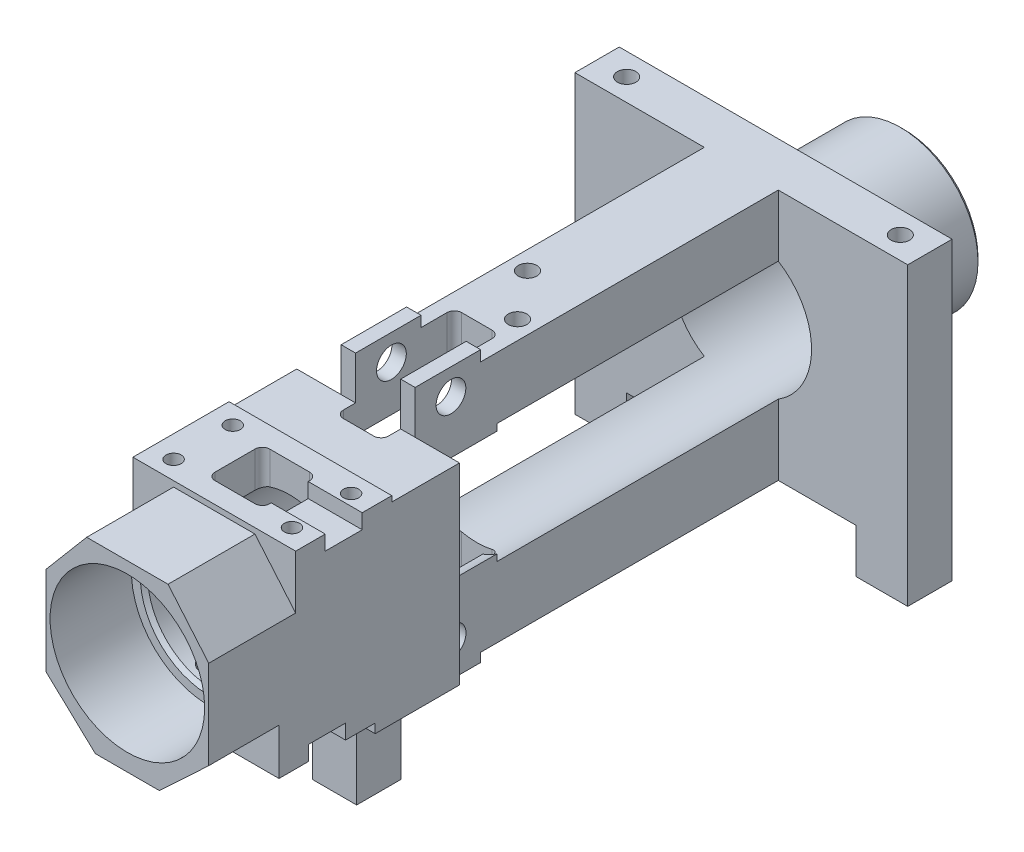
from build123d import *

# Parameters (mm, degrees)
SKETCH_1_R                   = 10.5
EXTRUDE_1_DEPTH              = 16
SKETCH_2_W                   = 45
SKETCH_2_H                   = 40
EXTRUDE_2_DEPTH              = 6
SKETCH_3_W                   = 10
SKETCH_3_H                   = 40
EXTRUDE_3_DEPTH              = 59
SKETCH_4_W                   = 22
SKETCH_4_H                   = 9.9
EXTRUDE_4_DEPTH              = 40
SKETCH_5_W                   = 8.85
SKETCH_5_H                   = 1.44
EXTRUDE_5_DEPTH              = 10
SKETCH_6_R                   = 8.75
CUT_EXTRUDE_1_DEPTH          = 88.316722339
SKETCH_7_W                   = 22
SKETCH_7_H                   = 4.4
SKETCH_7_H_2                 = 9.6
CUT_EXTRUDE_2_DEPTH          = 9.9
SKETCH_8_W                   = 6.1
SKETCH_8_H                   = 16
CUT_EXTRUDE_3_DEPTH          = 94.725789407
SKETCH_9_W                   = 10
SKETCH_9_H                   = 4.8
CUT_EXTRUDE_4_DEPTH          = 13.35
SKETCH_10_W                  = 31
SKETCH_10_H                  = 6
CUT_EXTRUDE_5_DEPTH          = 29.4
HOLE_WIZARD_M3_1_D           = 2.5
HOLE_WIZARD_M3_1_DEPTH       = 5
HOLE_WIZARD_M3_1_TIP         = 0.751075774
CUT_EXTRUDE_6_REACH          = 90.737
SKETCH_14_R                  = 2.01
SKETCH_14_R_2                = 2.03
HOLE_WIZARD_M3_2_D           = 2.5
HOLE_WIZARD_M3_2_DEPTH       = 5
HOLE_WIZARD_M3_2_TIP         = 0.751075774
SKETCH_18_R                  = 9.5
CUT_EXTRUDE_7_DEPTH          = 60
CHAMFER_1_SIZE               = 0.5
FILLET_1_R                   = 1
FILLET_2_R                   = 1
SKETCH_24_W                  = 10
SKETCH_24_H                  = 16.85
CUT_EXTRUDE_8_DEPTH          = 6
EXTRUDE_START                = 24
SKETCH_25_W                  = 22
SKETCH_25_H                  = 26
SKETCH_25_R                  = 8.75
EXTRUDE_8_DEPTH              = 24
SKETCH_26_R                  = 10.45
CUT_EXTRUDE_9_DEPTH          = 11
CHAMFER_5_SIZE               = 0.5
SKETCH_27_W                  = 6
SKETCH_27_H                  = 6
SKETCH_27_R                  = 1.2
EXTRUDE_9_DEPTH              = 9.6
HOLE_WIZARD_M3_5_D           = 2.5
HOLE_WIZARD_M3_5_DEPTH       = 9.6
HOLE_WIZARD_M3_5_TIP         = 0.751075774
SKETCH_41_W                  = 22
SKETCH_41_H                  = 13
SKETCH_41_R                  = 1
EXTRUDE_9959_DEPTH           = 0.75
CUT_EXTRUDE_START            = -12
CUT_EXTRUDE_10346_DEPTH      = 12
HOLE_WIZARD_10393_D          = 2.05
HOLE_WIZARD_10393_DEPTH      = 6.2
HOLE_WIZARD_10393_TIP        = 0.615882135
SKETCH_51_W                  = 7.3
SKETCH_51_H                  = 5
CUT_EXTRUDE_11630_DEPTH      = 2
SKETCH_47_R                  = 1
CUT_EXTRUDE_12263_DEPTH      = 1.25
CUT_EXTRUDE_12654_REACH      = 114.005
CUT_EXTRUDE_12654_END_RADIUS = 8.75
HOLE_WIZARD_12700_D          = 2.05
HOLE_WIZARD_12700_DEPTH      = 6.35
HOLE_WIZARD_12700_TIP        = 0.615882135
CUT_EXTRUDE_13929_DEPTH      = 112.655712348
CUT_EXTRUDE_13929_DEPTH_BACK = 2
SKETCH_52_W                  = 7.3
SKETCH_52_H                  = 5
CUT_EXTRUDE_1_2_DEPTH        = 9.5
CUT_EXTRUDE_2_2_DEPTH        = 2.25


with BuildPart() as part:
    # 草图1 → 凸台-拉伸1 (new body)
    with BuildSketch(Plane.XY):
        Circle(SKETCH_1_R)
    extrude(amount=EXTRUDE_1_DEPTH)

    # 草图2 → 凸台-拉伸2 (add)
    with BuildSketch(Plane.XY.offset(16)):
        with Locations((0, -3.6)):
            Rectangle(SKETCH_2_W, SKETCH_2_H)
    extrude(amount=EXTRUDE_2_DEPTH)

    # 草图3 → 凸台-拉伸3 (add)
    with BuildSketch(Plane.XY.offset(22)):
        with Locations((0, -3.6)):
            Rectangle(SKETCH_3_W, SKETCH_3_H)
    extrude(amount=EXTRUDE_3_DEPTH)

    # 草图4 → 凸台-拉伸4 (add)
    with BuildSketch(Plane.XZ.offset(23.6)):
        with Locations((0, 76.05)):
            Rectangle(SKETCH_4_W, SKETCH_4_H)
    extrude(amount=-EXTRUDE_4_DEPTH)

    # 草图5 → 凸台-拉伸5 (add)
    with BuildSketch(Plane(origin=(5, 0, 0), x_dir=(0, 0, -1), z_dir=(1, 0, 0))):
        with Locations((-66.675, 17.12)):
            Rectangle(SKETCH_5_W, SKETCH_5_H)
    extrude(amount=-EXTRUDE_5_DEPTH)

    # 草图6 → Cut-Extrude 1 (cut, through all)
    with BuildSketch(Plane.XY.offset(81)):
        Circle(SKETCH_6_R)
    extrude(amount=-CUT_EXTRUDE_1_DEPTH, mode=Mode.SUBTRACT)

    # 草图7 → Cut-Extrude 2 (cut)
    with BuildSketch(Plane.XY.offset(81)):
        with Locations((0, 14.2)):
            Rectangle(SKETCH_7_W, SKETCH_7_H)
        with Locations((0, -18.8)):
            Rectangle(SKETCH_7_W, SKETCH_7_H_2)
    extrude(amount=-CUT_EXTRUDE_2_DEPTH, mode=Mode.SUBTRACT)

    # 草图8 → 切除-拉伸3 (cut, through all)
    with BuildSketch(Plane(origin=(0, 17.84, 0), x_dir=(1, 0, 0), z_dir=(0, 1, 0))):
        with Locations((0, -65.75)):
            Rectangle(SKETCH_8_W, SKETCH_8_H)
    extrude(amount=-CUT_EXTRUDE_3_DEPTH, mode=Mode.SUBTRACT)

    # 草图9 → 切除-拉伸4 (cut)
    with BuildSketch(Plane.XY.offset(71.1)):
        with Locations((0, -21.2)):
            Rectangle(SKETCH_9_W, SKETCH_9_H)
    extrude(amount=-CUT_EXTRUDE_4_DEPTH, mode=Mode.SUBTRACT)

    # 草图10 → 切除-拉伸5 (cut)
    with BuildSketch(Plane(origin=(0, 0, 16), x_dir=(-1, 0, 0), z_dir=(0, 0, -1))):
        with Locations((0, -20.6)):
            Rectangle(SKETCH_10_W, SKETCH_10_H)
    extrude(amount=-CUT_EXTRUDE_5_DEPTH, mode=Mode.SUBTRACT)

    # M3 螺纹孔1
    with Locations(Plane(origin=(0, -23.6, 0), x_dir=(-1, 0, 0), z_dir=(0, -1, 0))):
        with Locations((-18.5, -19), (18.5, -19), (-2.5, -48.4), (2.5, -54.75)):
            Hole(HOLE_WIZARD_M3_1_D / 2, depth=HOLE_WIZARD_M3_1_DEPTH)
            with Locations((0, 0, -(HOLE_WIZARD_M3_1_DEPTH + HOLE_WIZARD_M3_1_TIP / 2))):  # 118° drill point
                Cone(0, HOLE_WIZARD_M3_1_D / 2, HOLE_WIZARD_M3_1_TIP, mode=Mode.SUBTRACT)

    # 切除-拉伸6: up to this face of the body (flat: up to its plane)
    cut_extrude_6_end = Plane(part.part.faces().sort_by_distance((-5, 11.936289267, 47.101067212))[0])
    # 草图14 → 切除-拉伸6 (cut, up to the picked face)
    with BuildSketch(Plane(origin=(5, 0, 0), x_dir=(0, 0, -1), z_dir=(1, 0, 0)), mode=Mode.PRIVATE) as cut_extrude_6_sk1:
        with Locations(Location((-66.25, 14.34, 0), (0, 0, 90))):
            Circle(SKETCH_14_R)
    cut_extrude_6_tool1 = split(extrude(cut_extrude_6_sk1.sketch, amount=-CUT_EXTRUDE_6_REACH, mode=Mode.PRIVATE), bisect_by=cut_extrude_6_end, keep=Keep.BOTH, mode=Mode.PRIVATE)
    # 草图14 → 切除-拉伸6 (cut, up to the picked face)
    with BuildSketch(Plane(origin=(5, 0, 0), x_dir=(0, 0, -1), z_dir=(1, 0, 0)), mode=Mode.PRIVATE) as cut_extrude_6_sk2:
        with Locations(Location((-66.25, -14.34, 0), (0, 0, 90))):
            Circle(SKETCH_14_R_2)
    cut_extrude_6_tool2 = split(extrude(cut_extrude_6_sk2.sketch, amount=-CUT_EXTRUDE_6_REACH, mode=Mode.PRIVATE), bisect_by=cut_extrude_6_end, keep=Keep.BOTH, mode=Mode.PRIVATE)
    add(cut_extrude_6_tool1.solids().sort_by(Axis((5, 14.34, 66.25), (-1, 0, 0)))[0], mode=Mode.SUBTRACT)
    add(cut_extrude_6_tool2.solids().sort_by(Axis((5, -14.34, 66.25), (-1, 0, 0)))[0], mode=Mode.SUBTRACT)

    # M3 螺纹孔2
    with Locations(Plane(origin=(0, 16.4, 0), x_dir=(1, 0, 0), z_dir=(0, 1, 0))):
        with Locations((-18.5, -19), (18.5, -19), (-2.5, -48.4), (2.5, -54.75)):
            Hole(HOLE_WIZARD_M3_2_D / 2, depth=HOLE_WIZARD_M3_2_DEPTH)
            with Locations((0, 0, -(HOLE_WIZARD_M3_2_DEPTH + HOLE_WIZARD_M3_2_TIP / 2))):  # 118° drill point
                Cone(0, HOLE_WIZARD_M3_2_D / 2, HOLE_WIZARD_M3_2_TIP, mode=Mode.SUBTRACT)

    # 草图18 → 切除-拉伸7 (cut)
    with BuildSketch(Plane(origin=(0, 0, 0), x_dir=(-1, 0, 0), z_dir=(0, 0, -1))):
        Circle(SKETCH_18_R)
    extrude(amount=-CUT_EXTRUDE_7_DEPTH, mode=Mode.SUBTRACT)

    # 倒角1
    chamfer_1_edges = [part.edges().sort_by_distance(p)[0] for p in [
        (-10.5, 0, 0),
    ]]
    chamfer(chamfer_1_edges, length=CHAMFER_1_SIZE)

    # 圆角1
    fillet_1_edges = [part.edges().sort_by_distance(p)[0] for p in [
        (-10.5, 0, 16),
    ]]
    fillet(fillet_1_edges, radius=FILLET_1_R)

    # 圆角2
    fillet_2_edges = [part.edges().sort_by_distance(p)[0] for p in [
        (-3.05, 10.100609711, 73.75),
        (-3.05, -11.100609711, 73.75),
        (3.05, -11.100609711, 73.75),
        (3.05, 10.100609711, 73.75),
        (-3.05, -13.89854143, 57.75),
        (3.05, -13.89854143, 57.75),
        (3.05, 12.69854143, 57.75),
        (-3.05, 12.69854143, 57.75),
    ]]
    fillet(fillet_2_edges, radius=FILLET_2_R)

    # 草图24 → 切除-拉伸8 (cut)
    with BuildSketch(Plane(origin=(0, -23.6, 0), x_dir=(-1, 0, 0), z_dir=(0, -1, 0))):
        with Locations((0, -53.825)):
            Rectangle(SKETCH_24_W, SKETCH_24_H)
    extrude(amount=-CUT_EXTRUDE_8_DEPTH, mode=Mode.SUBTRACT)

    # 草图25 → 凸台-拉伸8 (add)
    with BuildSketch(Plane.XY.offset(81).offset(EXTRUDE_START)):
        with Locations((0, -1)):
            Rectangle(SKETCH_25_W, SKETCH_25_H)
        Circle(SKETCH_25_R, mode=Mode.SUBTRACT)
    extrude(amount=-EXTRUDE_8_DEPTH)

    # 草图26 → 切除-拉伸9 (cut)
    with BuildSketch(Plane.XY.offset(105)):
        Circle(SKETCH_26_R)
    extrude(amount=-CUT_EXTRUDE_9_DEPTH, mode=Mode.SUBTRACT)

    # 倒角5
    chamfer_5_edges = [part.edges().sort_by_distance(p)[0] for p in [
        (-8.75, 0, 94),
    ]]
    chamfer(chamfer_5_edges, length=CHAMFER_5_SIZE)

    # 草图27 → 凸台-拉伸9 (add)
    # profile 1 of 2: a face of its own
    with BuildSketch(Plane(origin=(0, -14, 0), x_dir=(-1, 0, 0), z_dir=(0, -1, 0))):
        with Locations((5.5, -79.5)):
            Rectangle(SKETCH_27_W, SKETCH_27_H)
        with Locations(Location((5.5, -79.5, 0), (0, 0, 270))):
            Circle(SKETCH_27_R, mode=Mode.SUBTRACT)
    # profile 2 of 2: a face of its own
    with BuildSketch(Plane(origin=(0, -14, 0), x_dir=(-1, 0, 0), z_dir=(0, -1, 0))):
        with Locations((-5.5, -79.5)):
            Rectangle(SKETCH_27_W, SKETCH_27_H)
        with Locations((-5.5, -79.5)):
            Circle(SKETCH_27_R, mode=Mode.SUBTRACT)
    extrude(amount=EXTRUDE_9_DEPTH)

    # M3 螺纹孔5
    with Locations(Plane(origin=(0, -23.6, 0), x_dir=(-1, 0, 0), z_dir=(0, -1, 0))):
        with Locations((-5.5, -79.5), (5.5, -79.5)):
            Hole(HOLE_WIZARD_M3_5_D / 2, depth=HOLE_WIZARD_M3_5_DEPTH)
            with Locations((0, 0, -(HOLE_WIZARD_M3_5_DEPTH + HOLE_WIZARD_M3_5_TIP / 2))):  # 118° drill point
                Cone(0, HOLE_WIZARD_M3_5_D / 2, HOLE_WIZARD_M3_5_TIP, mode=Mode.SUBTRACT)

    # 草图41 → Extrude 9959 (add)
    with BuildSketch(Plane(origin=(0, 12, 0), x_dir=(1, 0, 0), z_dir=(0, 1, 0))):
        with Locations((0, -86.75)):
            Rectangle(SKETCH_41_W, SKETCH_41_H)
        with Locations(Location((-8, -82.75, 0), (0, 0, 90))):
            Circle(SKETCH_41_R, mode=Mode.SUBTRACT)
        with Locations(Location((8, -82.75, 0), (0, 0, 90))):
            Circle(SKETCH_41_R, mode=Mode.SUBTRACT)
        with Locations(Location((-8, -90.75, 0), (0, 0, 90))):
            Circle(SKETCH_41_R, mode=Mode.SUBTRACT)
        with Locations(Location((8, -90.75, 0), (0, 0, 90))):
            Circle(SKETCH_41_R, mode=Mode.SUBTRACT)
        with BuildLine():
            Line((-2.7, -90.45), (2.7, -90.45))
            ThreePointArc((2.7, -90.45), (3.407106781, -90.157106781), (3.7, -89.45))
            Line((3.7, -89.45), (3.7, -84.05))
            ThreePointArc((3.7, -84.05), (3.407106781, -83.342893219), (2.7, -83.05))
            Line((2.7, -83.05), (-2.7, -83.05))
            ThreePointArc((-2.7, -83.05), (-3.407106781, -83.342893219), (-3.7, -84.05))
            Line((-3.7, -84.05), (-3.7, -89.45))
            ThreePointArc((-3.7, -89.45), (-3.407106781, -90.157106781), (-2.7, -90.45))
        make_face(mode=Mode.SUBTRACT)
    extrude(amount=EXTRUDE_9959_DEPTH)

    # 草图44 → Cut-Extrude 10346 (cut)
    with BuildSketch(Plane(origin=(0, 12, 0), x_dir=(1, 0, 0), z_dir=(0, 1, 0)).offset(CUT_EXTRUDE_START)):
        with BuildLine():
            Line((-2.7, -90.45), (2.7, -90.45))
            ThreePointArc((2.7, -90.45), (3.407106781, -90.157106781), (3.7, -89.45))
            Line((3.7, -89.45), (3.7, -84.05))
            ThreePointArc((3.7, -84.05), (3.407106781, -83.342893219), (2.7, -83.05))
            Line((2.7, -83.05), (-2.7, -83.05))
            ThreePointArc((-2.7, -83.05), (-3.407106781, -83.342893219), (-3.7, -84.05))
            Line((-3.7, -84.05), (-3.7, -89.45))
            ThreePointArc((-3.7, -89.45), (-3.407106781, -90.157106781), (-2.7, -90.45))
        make_face()
    extrude(amount=CUT_EXTRUDE_10346_DEPTH, mode=Mode.SUBTRACT)

    # Hole Wizard 10393
    with Locations(Plane(origin=(0, 12.75, 0), x_dir=(1, 0, 0), z_dir=(0, 1, 0))):
        with Locations((-8, -82.75), (8, -82.75), (8, -90.75), (-8, -90.75)):
            Hole(HOLE_WIZARD_10393_D / 2, depth=HOLE_WIZARD_10393_DEPTH)
            with Locations((0, 0, -(HOLE_WIZARD_10393_DEPTH + HOLE_WIZARD_10393_TIP / 2))):  # 118° drill point
                Cone(0, HOLE_WIZARD_10393_D / 2, HOLE_WIZARD_10393_TIP, mode=Mode.SUBTRACT)

    # 草图51 → Cut-Extrude 11630 (cut)
    with BuildSketch(Plane(origin=(0, 12.75, 0), x_dir=(1, 0, 0), z_dir=(0, 1, 0))):
        with Locations((7.35, -86.75)):
            Rectangle(SKETCH_51_W, SKETCH_51_H)
    extrude(amount=-CUT_EXTRUDE_11630_DEPTH, mode=Mode.SUBTRACT)

    # 草图47 → Cut-Extrude 12263 (cut)
    with BuildSketch(Plane(origin=(0, -14, 0), x_dir=(-1, 0, 0), z_dir=(0, -1, 0))):
        with BuildLine():
            Line((-11.5, -82.5), (11.5, -82.5))
            ThreePointArc((11.5, -82.5), (12.207106781, -82.792893219), (12.5, -83.5))
            Line((12.5, -83.5), (12.5, -94.5))
            ThreePointArc((12.5, -94.5), (12.207106781, -95.207106781), (11.5, -95.5))
            Line((11.5, -95.5), (-11.5, -95.5))
            ThreePointArc((-11.5, -95.5), (-12.207106781, -95.207106781), (-12.5, -94.5))
            Line((-12.5, -94.5), (-12.5, -83.5))
            ThreePointArc((-12.5, -83.5), (-12.207106781, -82.792893219), (-11.5, -82.5))
        make_face()
        with Locations(Location((-8, -85, 0), (0, 0, 180))):
            Circle(SKETCH_47_R, mode=Mode.SUBTRACT)
        with Locations(Location((8, -85, 0), (0, 0, 180))):
            Circle(SKETCH_47_R, mode=Mode.SUBTRACT)
        with Locations(Location((-8, -93, 0), (0, 0, 180))):
            Circle(SKETCH_47_R, mode=Mode.SUBTRACT)
        with Locations(Location((8, -93, 0), (0, 0, 180))):
            Circle(SKETCH_47_R, mode=Mode.SUBTRACT)
        with BuildLine():
            Line((-2.7, -92.7), (2.7, -92.7))
            ThreePointArc((2.7, -92.7), (3.407106781, -92.407106781), (3.7, -91.7))
            Line((3.7, -91.7), (3.7, -86.3))
            ThreePointArc((3.7, -86.3), (3.407106781, -85.592893219), (2.7, -85.3))
            Line((2.7, -85.3), (-2.7, -85.3))
            ThreePointArc((-2.7, -85.3), (-3.407106781, -85.592893219), (-3.7, -86.3))
            Line((-3.7, -86.3), (-3.7, -91.7))
            ThreePointArc((-3.7, -91.7), (-3.407106781, -92.407106781), (-2.7, -92.7))
        make_face(mode=Mode.SUBTRACT)
    extrude(amount=-CUT_EXTRUDE_12263_DEPTH, mode=Mode.SUBTRACT)

    # Cut-Extrude 12654: up to this cylinder (the profile starts outside it)
    cut_extrude_12654_end = Plane(origin=(0, 0, 89), z_dir=(0, 0, 1)) * Cylinder(CUT_EXTRUDE_12654_END_RADIUS, 246.51, mode=Mode.PRIVATE)
    # 草图50 → Cut-Extrude 12654 (cut, up to the surface)
    with BuildSketch(Plane.XZ.offset(14), mode=Mode.PRIVATE) as cut_extrude_12654_sk1:
        with BuildLine():
            Line((-3.7, 91.7), (-3.7, 86.3))
            ThreePointArc((-3.7, 86.3), (-3.407106781, 85.592893219), (-2.7, 85.3))
            Line((-2.7, 85.3), (2.7, 85.3))
            ThreePointArc((2.7, 85.3), (3.407106781, 85.592893219), (3.7, 86.3))
            Line((3.7, 86.3), (3.7, 91.7))
            ThreePointArc((3.7, 91.7), (3.407106781, 92.407106781), (2.7, 92.7))
            Line((2.7, 92.7), (-2.7, 92.7))
            ThreePointArc((-2.7, 92.7), (-3.407106781, 92.407106781), (-3.7, 91.7))
        make_face()
    cut_extrude_12654_tool1 = extrude(cut_extrude_12654_sk1.sketch, amount=-CUT_EXTRUDE_12654_REACH, mode=Mode.PRIVATE) - cut_extrude_12654_end
    add(cut_extrude_12654_tool1.solids().sort_by_distance((0, -14, 89))[0], mode=Mode.SUBTRACT)

    # Hole Wizard 12700
    with Locations(Plane(origin=(0, -14, 0), x_dir=(-1, 0, 0), z_dir=(0, -1, 0))):
        with Locations((-8, -85), (8, -85), (8, -93), (-8, -93)):
            Hole(HOLE_WIZARD_12700_D / 2, depth=HOLE_WIZARD_12700_DEPTH)
            with Locations((0, 0, -(HOLE_WIZARD_12700_DEPTH + HOLE_WIZARD_12700_TIP / 2))):  # 118° drill point
                Cone(0, HOLE_WIZARD_12700_D / 2, HOLE_WIZARD_12700_TIP, mode=Mode.SUBTRACT)

    # 草图52 → Cut-Extrude 13929 (cut, two sides: drawn at the far end of the back side and taken through both)
    with BuildSketch(Plane.XZ.offset(12.75).offset(-CUT_EXTRUDE_13929_DEPTH_BACK)):
        with Locations((7.35, 89)):
            Rectangle(SKETCH_52_W, SKETCH_52_H)
    extrude(amount=CUT_EXTRUDE_13929_DEPTH + CUT_EXTRUDE_13929_DEPTH_BACK, mode=Mode.SUBTRACT)

    # 草图53 → Cut-Extrude 1 2 (cut)
    with BuildSketch(Plane.XY.offset(105)):
        Polygon((4.333333333, -12.75), (0, -12.75), (0, -14), (3, -14), align=None)
        Polygon((0, -12.75), (-4.333333333, -12.75), (-3, -14), (0, -14), align=None)
        Polygon((11, -14), (11, -6.5), (4.333333333, -12.75), (3, -14), align=None)
        Polygon((-4.333333333, -12.75), (-11, -6.5), (-11, -14), (-3, -14), align=None)
        Polygon((11, 12), (5.5, 12), (11, 5.5), align=None)
        Polygon((-11, 5.5), (-5.5, 12), (-11, 12), align=None)
    extrude(amount=-CUT_EXTRUDE_1_2_DEPTH, mode=Mode.SUBTRACT)

    # 草图54 → Cut-Extrude 2 2 (cut)
    with BuildSketch(Plane.XY.offset(95.5)):
        Polygon((11, 12), (5.5, 12), (11, 5.5), align=None)
        Polygon((-11, 12), (-11, 5.5), (-5.5, 12), align=None)
    extrude(amount=-CUT_EXTRUDE_2_2_DEPTH, mode=Mode.SUBTRACT)


solid = part.part
